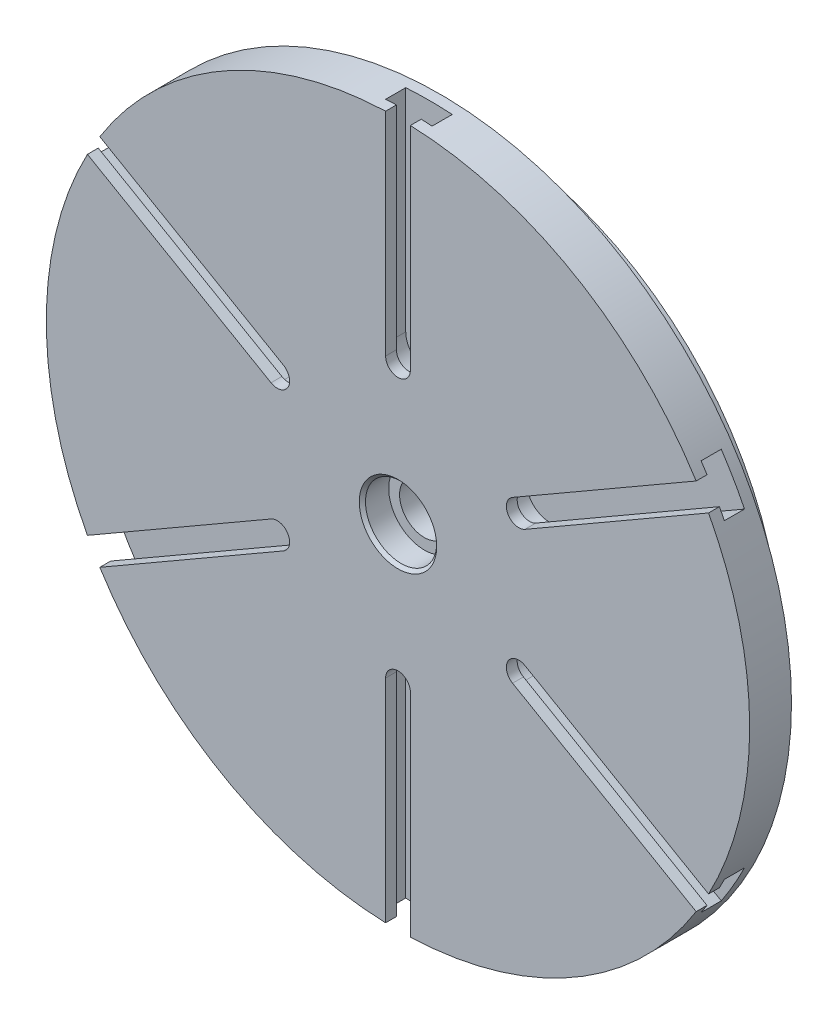
from build123d import *

# Parameters (mm, degrees)
SKETCH2_R          = 23
CUT_EXTRUDE1_DEPTH = 17
SKETCH3_R          = 16
CUT_EXTRUDE2_DEPTH = 606.281099986
CHAMFER1_SIZE      = 2
CUT_EXTRUDE3_DEPTH = 20
CUT_EXTRUDE4_DEPTH = 13
CIRPATTERN1_COUNT  = 6


with BuildPart() as part:
    # Sketch1 → Revolve1 (revolve)
    with BuildSketch(Plane(origin=(0, 318.5, 0), x_dir=(-1, 0, 0), z_dir=(0, -1, 0)), mode=Mode.PRIVATE) as revolve1_sk:
        Polygon((176, 77.5), (176, 87.5), (30, 87.5), (26, 174.5), (0, 174.5), (0, 26.1), (227, 26.1), (227, 53.1), (222, 53.1), (222, 50.1), (219, 50.1), (219, 51.1), (199, 51.1), (199, 50.1), (196, 50.1), (196, 51.1), (196, 77.5), align=None)
    revolve(revolve1_sk.sketch.rotate(Axis((0, 318.5, 0), (0, 0, -1)), 180), axis=Axis((0, 318.5, 0), (0, 0, -1)))

    # Sketch2 → Cut-Extrude1 (cut)
    with BuildSketch(Plane.XY.offset(-26.1)):
        with Locations((0, 318.5)):
            Circle(SKETCH2_R)
    extrude(amount=-CUT_EXTRUDE1_DEPTH, mode=Mode.SUBTRACT)

    # Sketch3 → Cut-Extrude2 (cut, through all)
    with BuildSketch(Plane.XY.offset(-43.1)):
        with Locations((0, 318.5)):
            Circle(SKETCH3_R)
    extrude(amount=-CUT_EXTRUDE2_DEPTH, mode=Mode.SUBTRACT)

    # Chamfer1
    chamfer1_edges = [part.edges().sort_by_distance(p)[0] for p in [
        (-23, 318.5, -26.1),
    ]]
    chamfer(chamfer1_edges, length=CHAMFER1_SIZE)

    # Sketch4 → Cut-Extrude3 (cut)
    with BuildSketch(Plane.XY.offset(-26.1)):
        with BuildLine():
            Line((-8, 606.712422614), (-8, 408.5))
            ThreePointArc((-8, 408.5), (0, 400.5), (8, 408.5))
            Line((8, 408.5), (8, 606.712422614))
            Line((8, 606.712422614), (-8, 606.712422614))
        make_face()
    cut_extrude3 = extrude(amount=-CUT_EXTRUDE3_DEPTH, mode=Mode.SUBTRACT)

    # Sketch5 → Cut-Extrude4 (cut)
    with BuildSketch(Plane.XY.offset(-33.1)):
        with BuildLine():
            Line((-15, 626.113520772), (-15, 408.5))
            ThreePointArc((-15, 408.5), (0, 393.5), (15, 408.5))
            Line((15, 408.5), (15, 626.113520772))
            Line((15, 626.113520772), (-15, 626.113520772))
        make_face()
    cut_extrude4 = extrude(amount=-CUT_EXTRUDE4_DEPTH, mode=Mode.SUBTRACT)

    # CirPattern1: Cut-Extrude3, Cut-Extrude4 ×6 about axis
    cirpattern1_axis = Axis((0, 318.5, 0), (0, 0, 1))
    add([cut_extrude3.rotate(cirpattern1_axis, i * 360 / CIRPATTERN1_COUNT) for i in range(1, CIRPATTERN1_COUNT)], mode=Mode.SUBTRACT)
    add([cut_extrude4.rotate(cirpattern1_axis, i * 360 / CIRPATTERN1_COUNT) for i in range(1, CIRPATTERN1_COUNT)], mode=Mode.SUBTRACT)


solid = part.part
